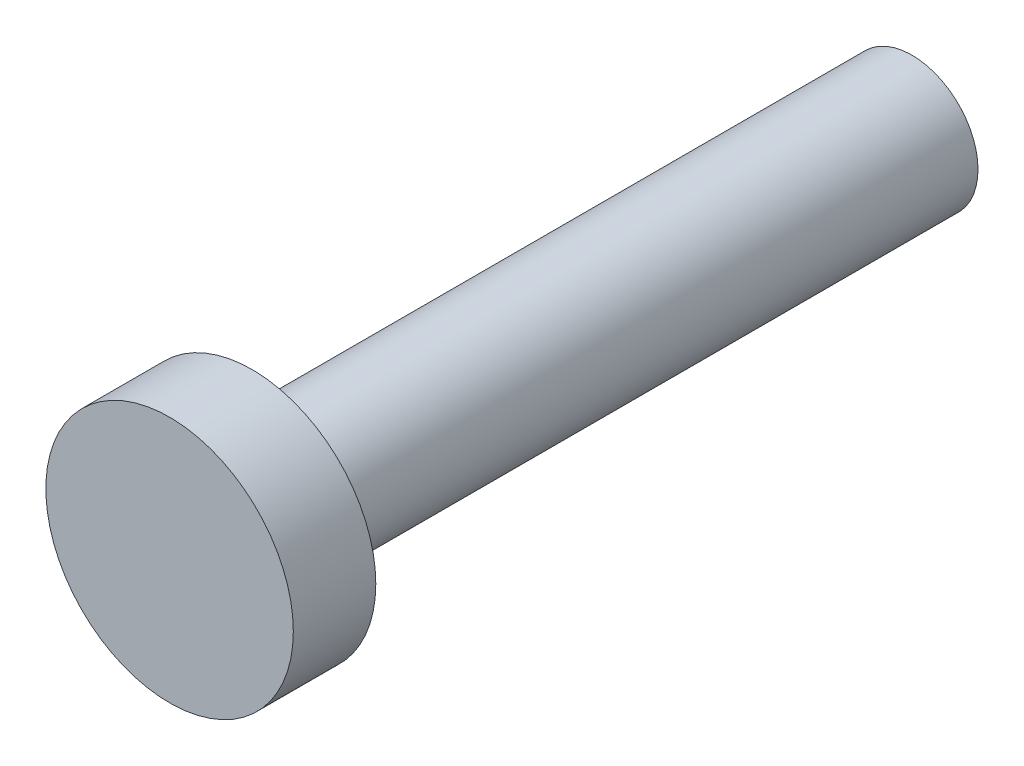
from build123d import *

# Parameters (mm, degrees)
SKETCH1_R           = 4
BOSS_EXTRUDE1_DEPTH = 40
SKETCH2_R           = 7.5
BOSS_EXTRUDE2_DEPTH = 5


with BuildPart() as part:
    # Sketch1 → Boss-Extrude1 (new body)
    with BuildSketch(Plane.XY):
        Circle(SKETCH1_R)
    extrude(amount=BOSS_EXTRUDE1_DEPTH)

    # Sketch2 → Boss-Extrude2 (add)
    with BuildSketch(Plane.XY.offset(40)):
        Circle(SKETCH2_R)
    extrude(amount=BOSS_EXTRUDE2_DEPTH)


solid = part.part
